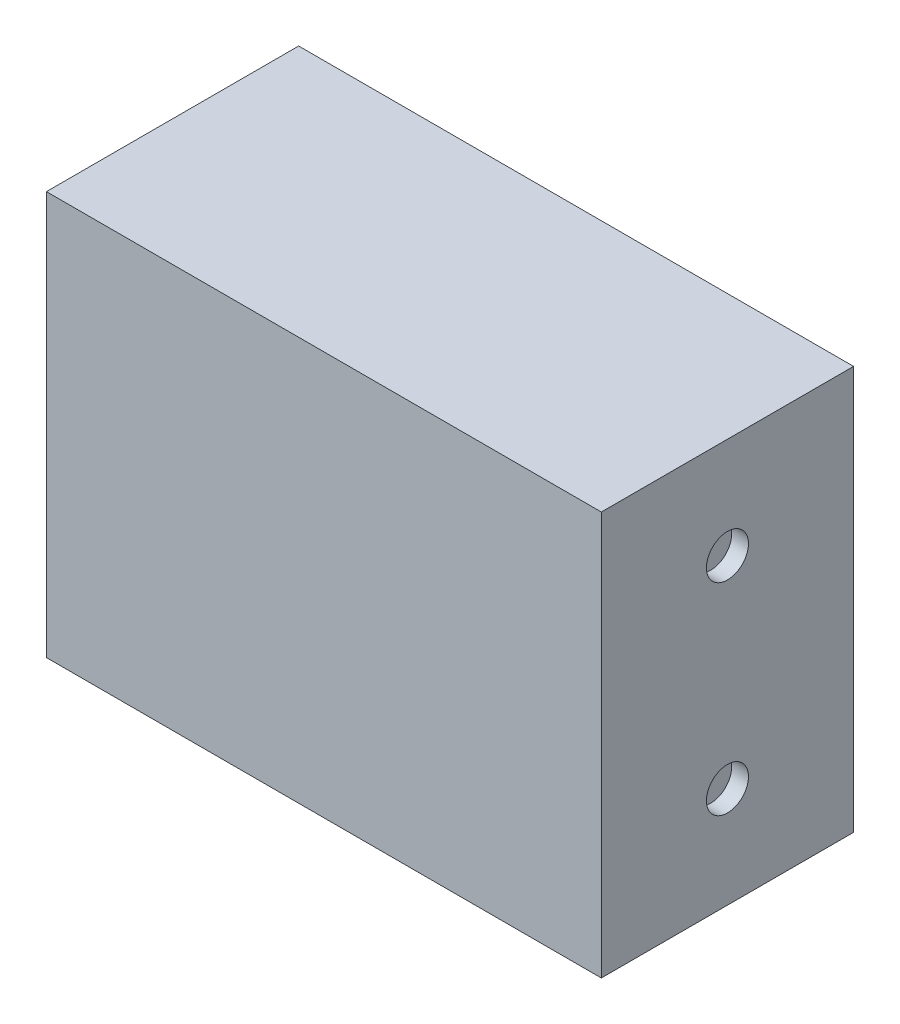
SolidWorks part; units mm, degrees
ref_plane "前视基准面" through (0, 0, 0) normal (0, 0, 1) x (1, 0, 0)
ref_plane "上视基准面" through (0, 0, 0) normal (0, 1, 0) x (1, 0, 0)
ref_plane "右视基准面" through (0, 0, 0) normal (1, 0, 0) x (0, 0, -1)
sketch "草图1" plane through (0, 0, 0) normal (0, 0, 1) x (1, 0, 0)
  line L1 (-165, 120) -> (165, 120)
  line L2 (-165, 120) -> (-165, -120)
  line L3 (-165, -120) -> (165, -120)
  line L4 (165, 120) -> (165, -120)
  line L5 (-165, 120) -> (165, -120) construction
  line L6 (-165, -120) -> (165, 120) construction
  point P0 (0, 0)
  dimension "D1" = 330
  dimension "D2" = 240
extrude "凸台-拉伸1" add sketch "草图1" along normal blind 150
sketch "草图2" plane through (165, 0, 0) normal (1, 0, 0) x (0, 0, -1)
  line L0 (-75, 120) -> (-75, -120) construction
  line L1 (-150, 120) -> (0, 120) construction
  line L2 (-150, -120) -> (0, -120) construction
  circle A0 centre (-75, 60) radius 12.5
  circle A1 centre (-75, -60) radius 12.5
  dimension "D1" = 25
  dimension "D2" = 25
  dimension "D3" = 60
  dimension "D4" = 60
extrude "切除-拉伸1" cut sketch "草图2" against normal blind 10
sketch "草图3" plane through (-165, 0, 0) normal (-1, 0, 0) x (0, 0, 1)
  line L0 (40, 80) -> (110, 80) construction
  line L1 (110, 80) -> (110, -80) construction
  line L2 (110, -80) -> (40, -80) construction
  line L3 (40, -80) -> (40, 80) construction
  line L4 (150, 120) -> (0, 120) construction
  line L5 (150, -120) -> (0, -120) construction
  line L6 (0, 120) -> (0, -120) construction
  line L7 (150, 120) -> (150, -120) construction
  circle A0 centre (40, 80) radius 2.75
  circle A1 centre (110, 80) radius 2.75
  circle A2 centre (110, -80) radius 2.75
  circle A3 centre (40, -80) radius 2.75
  dimension "D1" = 5.5
  dimension "D2" = 5.5
  dimension "D3" = 5.5
  dimension "D4" = 5.5
  dimension "D5" = 40
  dimension "D6" = 40
  dimension "D7" = 40
  dimension "D8" = 40
extrude "切除-拉伸2" cut sketch "草图3" against normal blind 10
